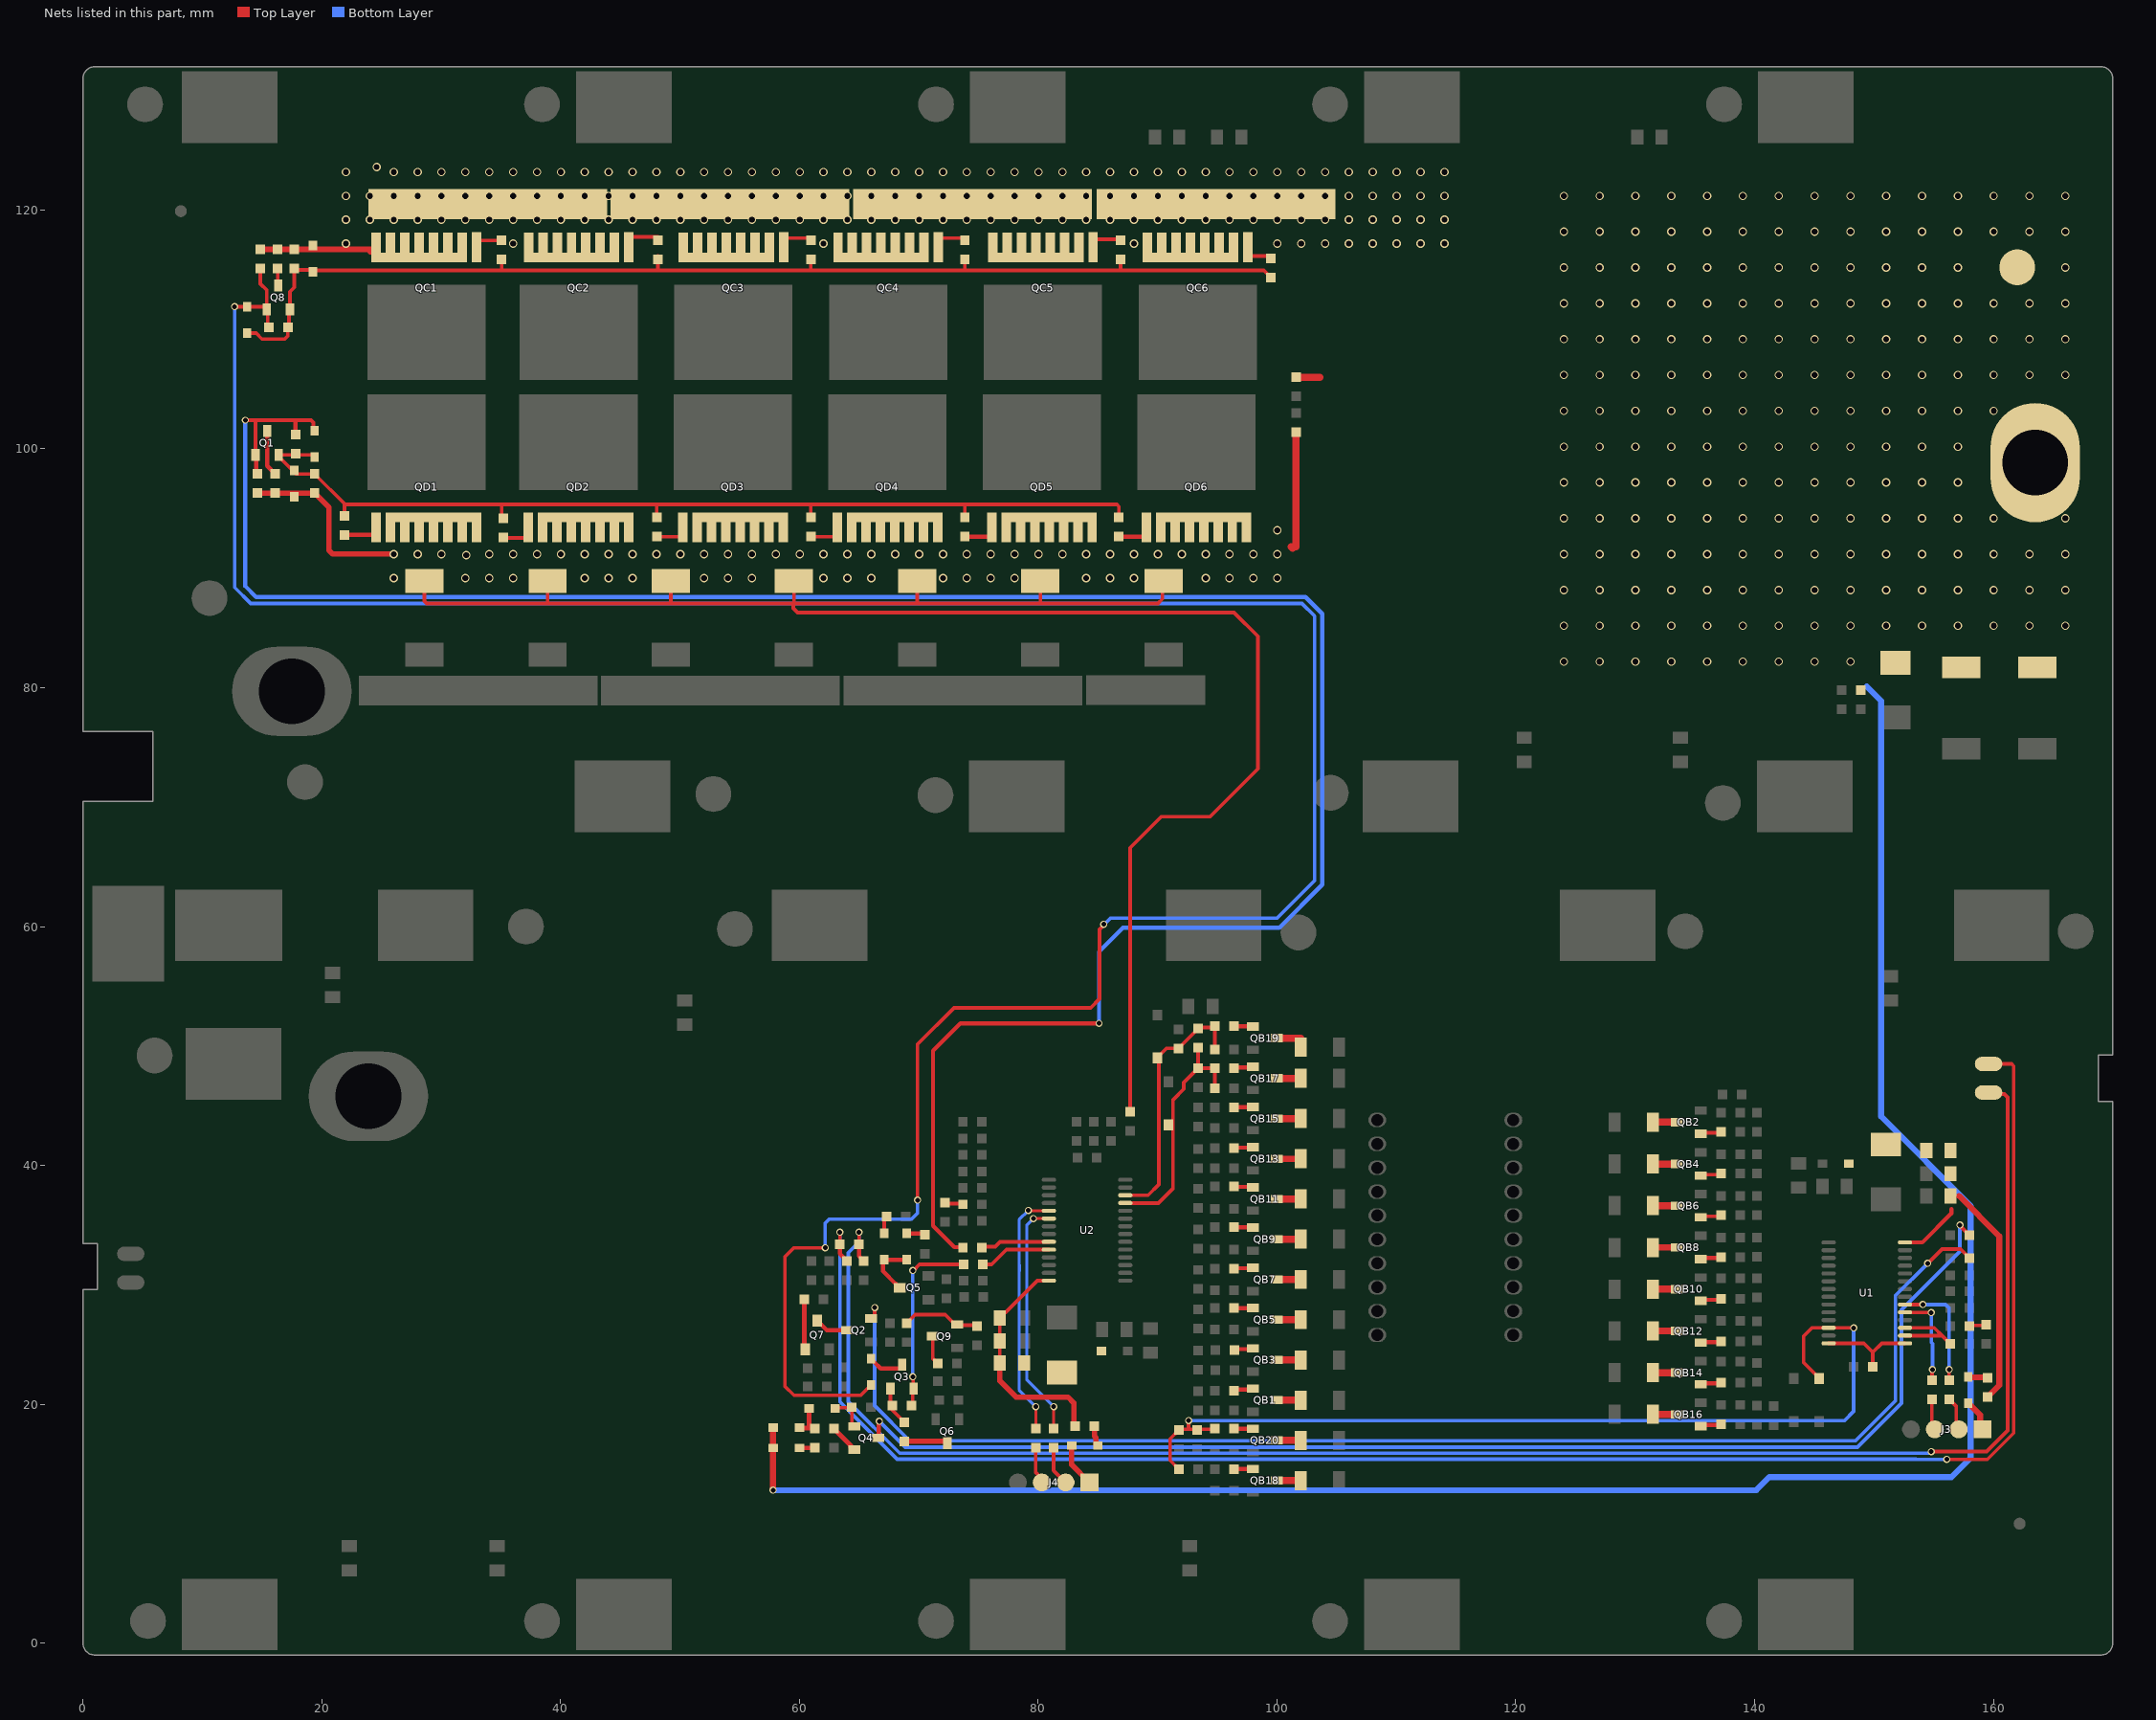
[diagram p0: the nets of this part, all layers, seen from the top]
# Altium PCB MISC82749.PcbDoc (part 3 of 4)
Units mm, origin at the board's own origin, x right, y up, seen from the top; angles counter-clockwise.
Board outline 170 x 133 mm, 2 copper layers (Top Layer, Bottom Layer); 262 components, 170 nets, 783 pads, 1052 vias.

## Via types
v1: diameter 0.7, hole 0.5, Top Layer to Bottom Layer, tented both sides, 953 vias
v2: diameter 0.6, hole 0.4, Top Layer to Bottom Layer, tented both sides, 99 vias

## Nets (pads, with @x,y where several pads share a name; then routed paths per layer and width w, separated by ;. In a path a pad name is that pad's centre, name@x,y a point inside that pad or via, vN(x,y) a via of type N, cw(c..) or ccw(c..) an arc to the next point about the centre after c; other vN are vias at no path point) (continued)
NetC45_2: C45.2 QD1.2 QD2.2 QD3.2 QD4.2 QD5.2 QD6.2 R30.2 R40.2 R41.2 R43.2 RS1.2 RS2.2 RS3.2 RS4.2 RS5.2 RS6.2 RS7.2 Z1.2 | length 186.9
  Top Layer w0.3: RS7.2@28.6,88.95 28.6,87.255 28.805,87.05 39.053,87.05 ; RS6.2@38.917,88.95 38.917,87.186 39.053,87.05 ; RS5.2@49.233,88.95 49.233,87.117 49.3,87.05 ; RS4.2@59.55,88.95 59.55,87.1 59.5,87.05 ; RS3.2@69.867,88.95 69.867,87.183 70,87.05 ; RS2.2@80.183,88.95 80.183,87.067 80.2,87.05 ; R30.2@87.7,44.5 87.7,66.593 90.307,69.2 94.4,69.2 98.4,73.2 98.4,84.3 96.4,86.3 59.85,86.3 59.5,86.65 59.5,87.05 ; RS1.2@90.5,88.95 90.407,88.857 90.407,87.428 90.03,87.05 80.2,87.05 ; 39.053,87.05 49.3,87.05 ; 49.3,87.05 59.5,87.05 ; 59.5,87.05 70,87.05 ; 70,87.05 80.2,87.05
  Top Layer w0.45: R40.2@14.6,96.3 R41.2@16.1,96.3 R43.2@19.4,96.3 20.6,95.1 20.6,91.5 20.9,91.2 v1@25.7,91.2
  Top Layer w0.6: 101.2,91.8 101.3,91.7 ; 101.6,91.8 C45.2@101.6,101.4
  other v1: 26.027,89.182 32.028,89.182 34.028,89.182 36.028,89.182 42.028,89.182 44.028,89.182 46.028,89.182 52.028,89.182 54.028,89.182 56.028,89.182 62.028,89.182 64.028,89.182 66.028,89.182 72.028,89.182 74.028,89.182 76.028,89.182 78.028,89.182 84.028,89.182 86.028,89.182 88.028,89.182 94.028,89.182 96.028,89.182 98.028,89.182 100.028,89.182 32.1,91.1 26.027,91.182 28.027,91.182 30.027,91.182 34.028,91.182 36.028,91.182 38.028,91.182 40.028,91.182 42.028,91.182 44.028,91.182 46.028,91.182 48.028,91.182 50.028,91.182 52.028,91.182 54.028,91.182 56.028,91.182 58.028,91.182 60.028,91.182 62.028,91.182 64.028,91.182 66.028,91.182 68.028,91.182 70.028,91.182 72.028,91.182 74.028,91.182 76.028,91.182 78.028,91.182 80.028,91.182 82.028,91.182 84.028,91.182 86.028,91.182 88.028,91.182 90.028,91.182 92.028,91.182 94.028,91.182 96.028,91.182 98.028,91.182 100.028,91.182 100.028,93.182
NetD1_1: D1.1 R26.2 TVS1.1
NetD2_1: D2.1 R27.2 TVS2.1
NetD7_1: D7.1 R34.2 | length 1.5
  Top Layer w0.5: D7.1@157.95,22.25 R34.2@159.45,22.25
NetD7_2: D7.2 J3.1 | length 2.7
  Top Layer w0.5: D7.2@157.9,20.1 157.9,20.05 158,19.95 158.05,19.95 158.893,19.107 158.893,18.057 J3.1@159.05,17.9
NetD8_1: D8.1 R37.2 | length 1.7
  Top Layer w0.45: R37.2@84.7,18.15 84.711,18.139 84.711,17.339 84.848,17.202 84.848,16.675 84.973,16.55 D8.1@85,16.55
NetD8_2: D8.2 J4.1 | length 3.7
  Top Layer w0.45: D8.2@82.8,16.55 82.8,14.95 J4.1@84.3,13.45
NetD11_1: D11.1 Q1.2 R42.2 R43.1 RD1.1 RD2.1 RD3.1 RD4.2 RD5.2 RD6.2 Z1.1 | length 82
  Top Layer w0.3: R42.2@17.8,99.6 R42.2@17.9,99.5 ; D11.1@19.4,99.3 19.2,99.5 R42.2@17.9,99.5 ; RD1.1@21.9,94.4 21.9,95.35 ; RD2.1@35.06,94.15 35.06,95.29 35,95.35 ; RD3.1@48.06,94.25 48.06,95.31 48.1,95.35 ; RD4.2@60.96,94.25 60.96,95.31 61,95.35 ; RD5.2@73.86,94.25 73.86,95.29 73.8,95.35 ; RD6.2@86.76,94.25 86.76,95.174 86.584,95.35 73.8,95.35 ; R42.2@17.9,99.5 Q1.2@16.4,99.5 16.4,99.35 17.85,97.9 R43.1@19.4,97.9 21.9,95.4 21.9,95.35 ; 21.9,95.35 35,95.35 ; 35,95.35 48.1,95.35 ; 48.1,95.35 61,95.35 ; 61,95.35 73.8,95.35
NetD11_2: D11.2 Q1.1 R33.2 R40.1 R42.1 | length 199.7
  Top Layer w0.35: v2(13.6,102.4) 17.8,102.4 ; 14.45,102.3 Q1.1@14.45,99.5 14.525,99.425 14.525,97.975 R40.1@14.6,97.9 ; R42.1@17.8,101.2 17.8,102.4 ; D11.2@19.4,101.5 19.303,101.597 19.303,102.195 19.097,102.4 17.8,102.4 ; R33.2@73.7,33.1 73.649,33.151 72.98,33.151 71.2,34.931 71.2,49.6 73.5,51.9 v2(85.1,51.9)
  Bottom Layer w0.35: v2(13.6,102.4) 13.6,88.5 14.5,87.6 102.4,87.6 103.8,86.2 103.8,63.5 100.2,59.9 87.1,59.9 85.1,57.9 v2(85.1,51.9)
NetD12_1: D12.1 D13.2 Q8.1 R53.1 R65.1 | length 234.2
  Top Layer w0.3: v2(12.7,111.9) 12.704,111.896 13.756,111.896 D13.2@13.76,111.892 15.185,111.892 Q8.1@15.385,111.692 ; R65.1@14.86,115.1 14.86,113.825 15.385,113.3 Q8.1@15.385,111.692 ; R53.1@15.56,110.192 15.472,110.279 15.472,111.588 Q8.1@15.385,111.676 Q8.1@15.385,111.692 ; v2(62.164,33.1) 59.538,33.1 58.8,32.362 58.8,21.5 59.55,20.75 65.15,20.75 65.75,21.35 65.8,21.35 66,21.55 D12.1@66,21.6 ; v2(69.9,37.1) 69.9,50.15 72.95,53.2 84.4,53.2 85.15,53.95 85.15,59.769 85.5,60.119 v2(85.5,60.2)
  Bottom Layer w0.3: v2(12.7,111.9) 12.7,88.4 14.05,87.05 102.1,87.05 103.15,86 103.15,63.85 100,60.7 86.061,60.7 85.561,60.2 v2(85.5,60.2) ; v2(62.164,33.1) 62.164,35.164 62.5,35.5 69.4,35.5 69.9,36 v2(69.9,37.1)
NetD12_2: D12.2 Q3.3 | length 3.2
  Top Layer w0.35: D12.2@66,23.8 66,23.75 66.175,23.575 66.225,23.575 66.8,23 68.425,23 68.6,23.175 Q3.3@68.6,23.316
NetD13_1: D13.1 Q8.2 R52.1 R53.2 RC1.1 RC2.2 RC3.2 RC4.1 RC5.1 RC6.1 Z3.1 | length 97.1
  Top Layer w0.3: D13.1@13.76,109.692 14.508,109.692 15,109.2 16.9,109.2 17.16,109.46 R53.2@17.16,110.192 17.247,110.279 17.247,111.588 Q8.2@17.335,111.676 17.335,113.155 17.7,113.52 R52.1@17.7,115.1 17.81,114.99 Z3.1@19.26,114.99 ; Z3.1@19.26,114.842 19.368,114.95 35.1,114.95 ; RC1.1@35.06,115.85 35.06,114.99 35.1,114.95 ; RC2.2@48.16,116.15 48.16,114.99 48.2,114.95 ; RC3.2@60.96,116.05 60.96,115.01 60.9,114.95 ; RC4.1@73.86,116.05 73.86,114.99 73.9,114.95 ; RC5.1@86.9,115.95 86.9,115.05 86.8,114.95 ; RC6.1@99.5,114.35 98.9,114.95 86.8,114.95 ; 35.1,114.95 48.2,114.95 ; 48.2,114.95 60.9,114.95 ; 60.9,114.95 73.9,114.95 ; 73.9,114.95 86.8,114.95
NetD14_1: D14.1 R55.1 | length 1.5
  Top Layer w0.35: D14.1@69,34.3 70.275,34.3 70.35,34.225 R55.1@70.35,34.1
NetD14_2: D14.2 D16.1 Q5.3 | length 4.8
  Top Layer w0.35: Q5.3@68.4,29.75 68.3,29.75 68.075,29.975 68.075,30.075 67,31.15 67,32.1 D16.1@67.1,32.1 D14.2@68.8,32.1
NetD15_2: D15.2 R58.1 Z2.2 | length 3
  Top Layer w0.4: D15.2@60,18.05 60.05,18 60.7,18 ; Z2.2@60.8,19.65 60.8,18.1 60.7,18 ; R58.1@61.3,17.95 61.25,18 60.7,18
NetD16_2: D16.2 R66.2 | length 1.4
  Top Layer w0.3: D16.2@67.1,34.3 R66.2@67.1,35.7
NetD17_2: D17.2 R57.1 | length 1.3
  Top Layer w0.35: D17.2@60,16.35 R57.1@61.3,16.35
NetJ3_2: J3.2 R35.2 | length 2.8
  Top Layer w0.3: R35.2@156.3,20.4 156.9,19.8 156.9,18.1 J3.2@157.1,17.9
NetJ3_3: J3.3 R36.2 | length 2.6
  Top Layer w0.3: R36.2@154.85,20.4 154.85,18.475 155.1,18.225 J3.3@155.1,17.9
NetJ4_2: J4.2 R38.2 | length 3.3
  Top Layer w0.3: R38.2@81.3,16.35 81.3,14.45 J4.2@82.3,13.45
NetJ4_3: J4.3 R39.2 | length 3.1
  Top Layer w0.3: R39.2@79.8,16.35 79.8,14.275 80.3,13.775 J4.3@80.3,13.45
NetQ1_3: Q1.3 R41.1 | length 3.9
  Top Layer w0.35: Q1.3@15.425,101.516 15.425,98.575 R41.1@16.1,97.9
NetQ2_2: Q2.2 R44.1 | length 114.3
  Top Layer w0.3: Q2.2@66,27.175 66.11,27.175 66.31,27.375 v2(66.31,28.09) ; v2(154.5,31.8) 155.7,33 157.25,33 R44.1@158,32.25
  Bottom Layer w0.3: v2(66.31,28.09) 66.31,19.883 69.243,16.95 148.457,16.95 151.8,20.293 151.8,29.1 v2(154.5,31.8)
NetQ2_3: Q2.3 Q7.3 | length 2.7
  Top Layer w0.35: Q7.3@61.5,27 61.5,26.9 61.725,26.675 61.825,26.675 62.3,26.2 Q2.3@63.8,26.2
NetQ3_1: Q3.1 R54.1 R56.1 | length 3.3
  Top Layer w0.3: Q3.1@67.625,21.3 67.625,19.675 R56.1@68.8,18.5
NetQ3_2: Q3.2 R32.2 R54.2 | length 15.8
  Top Layer w0.3: R54.2@69.4,19.9 69.488,19.988 69.488,21.388 69.538,21.438 69.538,22.263 v2(69.5,22.3) ; v2(69.5,31.2) 69.542,31.2 70.051,31.71 R32.2@73.76,31.71
  Bottom Layer w0.3: v2(69.5,22.3) v2(69.5,31.2)
NetQ4_1: Q4.1 R45.2 Z2.1 | length 3.1
  Top Layer w0.3: Z2.1@63,19.65 63.05,19.7 64.35,19.7 R45.2@64.4,19.75 64.4,18.35 Q4.1@64.6,18.15
NetQ4_2: Q4.2 R58.2 | length 2.5
  Top Layer w0.4: R58.2@62.9,17.95 64.3,16.55 64.3,16.35 64.45,16.2 Q4.2@64.6,16.2
NetQ4_3: Q4.3 R48.1 | length 107.6
  Top Layer w0.3: v2(157.2,35) 157.2,34.95 R48.1@158,34.15
  Top Layer w0.35: Q4.3@66.616,17.175 66.658,17.217 66.658,18.532 v2(66.7,18.574)
  Bottom Layer w0.3: v2(66.7,18.574) 68.874,16.4 148.614,16.4 152.3,20.086 152.3,27.9 157.2,32.8 v2(157.2,35)
NetQ6_3: Q6.3 R56.2 | length 3.7
  Top Layer w0.45: R56.2@68.815,16.9 72.275,16.9 72.4,16.775 Q6.3@72.4,16.734
NetQ7_1: Q7.1 R50.1 | length 3.7
  Top Layer w0.4: 60.4,25.144 R50.1@60.4,28.8
NetQ8_3: Q8.3 R61.1 | length 1.4
  Top Layer w0.3: R61.1@16.28,115.1 16.32,115.06 16.32,113.732 Q8.3@16.36,113.692
NetQ9_2: Q9.2 R59.1 R64.1 | length 6.6
  Top Layer w0.3: R59.1@69,26.8 69.7,27.5 72.225,27.5 73.05,26.675 Q9.2@73.2,26.675 ; Q9.2@73.2,26.613 74.838,26.613 R64.1@74.9,26.55
NetQ9_3: Q9.3 R62.2 | length 2.5
  Top Layer w0.3: Q9.3@71.184,25.7 71.184,23.816 R62.2@71.6,23.4
NetQB1_1: QB1.1 RB3.1 | length 1.7
  Top Layer w0.35: RB3.1@96.4,21.15 96.485,21.235 97.899,21.235 QB1.1@97.984,21.32
NetQB1_3: QB1.3 RB1.2 | length 2
  Top Layer w0.6: QB1.3@100,20.345 RB1.2@102,20.345
NetQB2_1: QB2.1 RB4.1 | length 1.8
  Top Layer w0.35: QB2.1@135.5,42.643 135.587,42.73 137.113,42.73 RB4.1@137.2,42.818
NetQB2_3: QB2.3 RB2.2 | length 2
  Top Layer w0.6: RB2.2@131.484,43.618 QB2.3@133.484,43.618
NetQB3_1: QB3.1 RB7.1 | length 1.6
  Top Layer w0.35: RB7.1@96.45,24.55 96.519,24.619 97.915,24.619 QB3.1@97.984,24.689
NetQB3_3: QB3.3 RB5.2 | length 2
  Top Layer w0.6: QB3.3@100,23.714 RB5.2@102,23.714
NetQB4_1: QB4.1 RB8.1 | length 1.8
  Top Layer w0.3: QB4.1@135.5,39.147 135.586,39.233 137.114,39.233 RB8.1@137.2,39.32
NetQB4_3: QB4.3 RB6.2 | length 2
  Top Layer w0.6: RB6.2@131.484,40.122 QB4.3@133.484,40.122
NetQB5_1: QB5.1 RB11.1 | length 1.6
  Top Layer w0.35: RB11.1@96.4,28.05 96.403,28.053 97.981,28.053 QB5.1@97.984,28.057
NetQB5_3: QB5.3 RB9.2 | length 2
  Top Layer w0.6: QB5.3@100,27.082 RB9.2@102,27.082
NetQB6_1: QB6.1 RB12.1 | length 1.8
  Top Layer w0.3: QB6.1@135.5,35.652 135.585,35.737 137.115,35.737 RB12.1@137.2,35.822
NetQB6_3: QB6.3 RB10.2 | length 2
  Top Layer w0.6: RB10.2@131.484,36.627 QB6.3@133.484,36.627
NetQB7_1: QB7.1 RB15.1 | length 1.6
  Top Layer w0.35: RB15.1@96.4,31.35 96.438,31.388 97.947,31.388 QB7.1@97.984,31.425
NetQB7_3: QB7.3 RB13.2 | length 2
  Top Layer w0.6: QB7.3@100,30.45 RB13.2@102,30.45
NetQB8_1: QB8.1 RB16.1 | length 1.8
  Top Layer w0.35: QB8.1@135.5,32.156 135.584,32.24 137.116,32.24 RB16.1@137.2,32.324
NetQB8_3: QB8.3 RB14.2 | length 2
  Top Layer w0.5: RB14.2@131.484,33.131 QB8.3@133.484,33.131
NetQB9_1: QB9.1 RB19.1 | length 1.6
  Top Layer w0.35: RB19.1@96.4,34.85 96.428,34.822 97.956,34.822 QB9.1@97.984,34.793
NetQB9_3: QB9.3 RB17.2 | length 2
  Top Layer w0.6: QB9.3@100,33.818 RB17.2@102,33.818
NetQB10_1: QB10.1 RB20.1 | length 1.8
  Top Layer w0.35: QB10.1@135.5,28.661 135.582,28.744 137.118,28.744 RB20.1@137.2,28.826
NetQB10_3: QB10.3 RB18.2 | length 2
  Top Layer w0.6: RB18.2@131.484,29.636 QB10.3@133.484,29.636
NetQB11_1: QB11.1 RB23.1 | length 1.6
  Top Layer w0.35: RB23.1@96.4,38.25 96.444,38.206 97.94,38.206 QB11.1@97.984,38.161
NetQB11_3: QB11.3 RB21.2 | length 2
  Top Layer w0.6: QB11.3@100,37.186 RB21.2@102,37.186
NetQB12_1: QB12.1 RB24.1 | length 1.7
  Top Layer w0.35: QB12.1@135.5,25.166 135.542,25.208 137.158,25.208 RB24.1@137.2,25.25
NetQB12_3: QB12.3 RB22.2 | length 2
  Top Layer w0.6: RB22.2@131.484,26.141 QB12.3@133.484,26.141
NetQB13_1: QB13.1 RB27.1 | length 1.6
  Top Layer w0.35: RB27.1@96.4,41.45 96.44,41.49 97.944,41.49 QB13.1@97.984,41.53
NetQB13_3: QB13.3 RB25.2 | length 2
  Top Layer w0.5: QB13.3@100,40.555 RB25.2@102,40.555
NetQB14_1: QB14.1 RB28.1 | length 1.8
  Top Layer w0.35: QB14.1@135.5,21.67 135.58,21.75 137.12,21.75 RB28.1@137.2,21.83
NetQB14_3: QB14.3 RB26.2 | length 2
  Top Layer w0.6: RB26.2@131.484,22.645 QB14.3@133.484,22.645
NetQB15_1: QB15.1 RB31.1 | length 1.6
  Top Layer w0.35: RB31.1@96.4,44.85 96.424,44.874 97.96,44.874 QB15.1@97.984,44.898
NetQB15_3: QB15.3 RB29.2 | length 2
  Top Layer w0.6: QB15.3@100,43.923 RB29.2@102,43.923
NetQB16_1: QB16.1 RB32.1 | length 1.8
  Top Layer w0.35: QB16.1@135.5,18.175 135.579,18.254 137.121,18.254 RB32.1@137.2,18.332
NetQB16_3: QB16.3 RB30.2 | length 2
  Top Layer w0.6: RB30.2@131.484,19.15 QB16.3@133.484,19.15
NetQB17_1: QB17.1 RB35.1 | length 1.6
  Top Layer w0.35: RB35.1@96.4,48.15 96.458,48.208 97.926,48.208 QB17.1@97.984,48.266
NetQB17_3: QB17.3 RB33.2 | length 2
  Top Layer w0.6: QB17.3@100,47.291 RB33.2@102,47.291
NetQB18_1: QB18.1 RB36.1 | length 1.6
  Top Layer w0.35: RB36.1@96.4,14.55 96.417,14.567 97.967,14.567 QB18.1@97.984,14.584
NetQB18_3: QB18.3 RB34.2 | length 2
  Top Layer w0.6: QB18.3@100,13.609 RB34.2@102,13.609
NetQB19_1: QB19.1 RB39.1 | length 1.6
  Top Layer w0.3: RB39.1@96.4,51.5 RB39.1@96.467,51.567
  Top Layer w0.35: RB39.1@96.467,51.567 96.542,51.642 97.976,51.642 QB19.1@97.984,51.634
NetQB19_3: QB19.3 RB37.2 | length 2
  Top Layer w0.6: QB19.3@100,50.659 RB37.2@102,50.659
NetQB20_1: QB20.1 RB40.1 | length 1.6
  Top Layer w0.35: RB40.1@96.4,17.95 96.401,17.951 97.983,17.951 QB20.1@97.984,17.952
NetQB20_3: QB20.3 RB38.2 | length 2
  Top Layer w0.6: QB20.3@100,16.977 RB38.2@102,16.977
NetQC1_1: QC1.1 RC1.2 | length 2.7
  Top Layer w0.3: QC1.1@32.76,116.888 32.76,117.2 33.01,117.45 RC1.2@35.06,117.45
NetQC2_1: QC2.1 RC2.1 | length 3.2
  Top Layer w0.3: QC2.1@45.72,116.888 45.72,117.5 45.97,117.75 RC2.1@48.16,117.75
NetQC3_1: QC3.1 RC3.1 | length 2.9
  Top Layer w0.3: QC3.1@58.68,116.888 58.68,117.4 58.93,117.65 RC3.1@60.96,117.65
NetQC4_1: QC4.1 RC4.2 | length 2.8
  Top Layer w0.3: QC4.1@71.64,116.888 71.64,117.4 71.89,117.65 RC4.2@73.86,117.65
NetQC5_1: QC5.1 RC5.2 | length 2.8
  Top Layer w0.3: QC5.1@84.6,116.888 84.6,117.3 84.85,117.55 RC5.2@86.9,117.55
NetQC6_1: QC6.1 RC6.2 | length 2.1
  Top Layer w0.35: QC6.1@97.492,116.15 99.3,116.15 RC6.2@99.5,115.95
NetQD1_1: QD1.1 RD1.2 | length 3.2
  Top Layer w0.3: QD1.1@24.36,93.35 QD1.1@24.36,93.412
  Top Layer w0.35: RD1.2@21.9,92.8 24.335,92.8 24.56,93.025 QD1.1@24.56,93.412
NetQD2_1: QD2.1 RD2.2 | length 3
  Top Layer w0.3: RD2.2@35.06,92.55 37.05,92.55 37.3,92.8 QD2.1@37.3,93.412
NetQD3_1: QD3.1 RD3.2 | length 2.8
  Top Layer w0.3: RD3.2@48.06,92.65 49.99,92.65 50.24,92.9 QD3.1@50.24,93.412
NetQD4_1: QD4.1 RD4.1 | length 2.8
  Top Layer w0.3: RD4.1@60.96,92.65 62.93,92.65 63.18,92.9 QD4.1@63.18,93.412
NetQD5_1: QD5.1 RD5.1 | length 2.9
  Top Layer w0.35: RD5.1@73.86,92.65 75.895,92.65 76.12,92.875 QD5.1@76.12,93.412
NetQD6_1: QD6.1 RD6.1 | length 2.9
  Top Layer w0.35: RD6.1@86.76,92.65 88.835,92.65 89.06,92.875 QD6.1@89.06,93.412
NetR28_2: R28.2 U1.14 U1.15 | length 8.2
  Top Layer w0.3: U1.14@146.2,25.1 149.15,25.1 149.9,24.35 ; R28.2@149.9,23.15 149.9,24.35 ; U1.15@152.6,25.1 150.65,25.1 149.9,24.35
NetR32_1: R32.1 U2.24 | length 6.4
  Top Layer w0.3: R32.1@75.619,31.45 R32.1@75.36,31.71 76.11,31.71 77.35,32.95 U2.24@80.9,32.95
NetR33_1: R33.1 U2.23 | length 5.8
  Top Layer w0.3: R33.1@75.3,33.1 75.4,33.2 76.4,33.2 76.8,33.6 U2.23@80.9,33.6
NetR67_1: R67.1 R70.2 SW1.1 | length 146.8
  Top Layer w0.254: R67.1@65.4,32 R67.1@65.627,31.773
  Top Layer w0.3: R70.2@65,33.4 v2(65,34.4) ; v2(154.8,16.038) 159.438,16.038 161.2,17.8 161.2,45.7 160.917,45.983 159.717,45.983 SW1.1@159.6,46.1
  Top Layer w0.35: R70.2@65,33.4 65,32.4 R67.1@65.4,32
  Bottom Layer w0.3: v2(65,34.4) 65,33.6 64.1,32.7 64.1,20.207 68.407,15.9 154.581,15.9 154.719,16.038 v2(154.8,16.038)
NetR68_2: R68.2 R70.1 SW1.2 | length 151
  Top Layer w0.3: R70.1@63.4,33.4 v2(63.4,34.4) ; v2(156.1,15.388) 156.088,15.4 156.1,15.4 156.112,15.388 159.495,15.388 161.7,17.593 161.7,48.324 161.524,48.5 SW1.2@159.6,48.5
  Top Layer w0.35: R70.1@63.4,33.4 63.4,32.6 R68.2@64,32
  Bottom Layer w0.3: v2(63.4,34.4) 63.4,20.2 64.95,18.65 64.95,18.643 68.193,15.4 153.5,15.4 153.512,15.388 v2(156.1,15.388)
NetR71_2: R71.2 U1.16 U1.17 | length 7.5
  Top Layer w0.3: U1.16@152.6,25.75 155.7,25.75 ; U1.17@152.6,26.4 155.05,26.4 155.7,25.75 ; R71.2@156.4,25.05 155.7,25.75
NetRT5_1: RT5.1 RT7.1 | length 1.4
  Top Layer w0.3: RT7.1@158,26.55 158.05,26.6 159.35,26.6 RT5.1@159.4,26.65
NetRT6_1: RT6.1 RT8.1 | length 1.5
  Top Layer w0.3: RT6.1@72.256,36.805 73.635,36.805 RT8.1@73.7,36.74
P-/C-: C41.1 C46.1 D9.2 D15.1 D17.1 pad.66@163.5,98.85 pad.82@33.9,120.5 pad.83@54.2,120.5 pad.84 pad.85 pad.86@162,115.2 QC1.2 QC2.2 QC3.2 QC4.2 QC5.2 QC6.2 R52.2 R61.2 R65.2 TVS3.1 TVS4.1 Z3.2 | length 188.7
  Top Layer w0.5: R65.2@14.86,116.7 R61.2@16.28,116.7 R52.2@17.7,116.7 24.41,116.7 24.56,116.85 QC1.2@24.56,117.25 ; 24.068,116.508 24.21,116.65 QC1.2@24.41,116.65 ; v2(57.8,12.8) D17.1@57.8,16.35 D15.1@57.8,18.05 ; C46.1@101.6,106 C46.1@101.75,106.15 ; D9.2@151.05,82.85 D9.2@151.8,82.1
  Top Layer w0.6: C46.1@101.6,106 103.2,106 103.6,106
  Bottom Layer w0.5: v2(57.8,12.8) 140.139,12.8 141.239,13.9 156.5,13.9 158.1,15.5 158.1,36.6 150.6,44.1 150.6,78.9 149.4,80.1
  other v1: 124.027,82.182 127.027,82.182 130.027,82.182 133.027,82.182 136.027,82.182 139.027,82.182 142.027,82.182 145.027,82.182 148.027,82.182 124.027,85.182 127.027,85.182 130.027,85.182 133.027,85.182 136.027,85.182 139.027,85.182 142.027,85.182 145.027,85.182 148.027,85.182 151.027,85.182 154.027,85.182 157.027,85.182 160.027,85.182 163.027,85.182 166.027,85.182 124.027,88.182 127.027,88.182 130.027,88.182 133.027,88.182 136.027,88.182 139.027,88.182 142.027,88.182 145.027,88.182 148.027,88.182 151.027,88.182 154.027,88.182 157.027,88.182 160.027,88.182 163.027,88.182 166.027,88.182 124.027,91.182 127.027,91.182 130.027,91.182 133.027,91.182 136.027,91.182 139.027,91.182 142.027,91.182 145.027,91.182 148.027,91.182 151.027,91.182 154.027,91.182 157.027,91.182 160.027,91.182 163.027,91.182 166.027,91.182 124.027,94.182 127.027,94.182 130.027,94.182 133.027,94.182 136.027,94.182 139.027,94.182 142.027,94.182 145.027,94.182 148.027,94.182 151.027,94.182 154.027,94.182 157.027,94.182 160.027,94.182 166.027,94.182 124.027,97.182 127.027,97.182 130.027,97.182 133.027,97.182 136.027,97.182 139.027,97.182 142.027,97.182 145.027,97.182 148.027,97.182 151.027,97.182 154.027,97.182 157.027,97.182 124.027,100.182 127.027,100.182 130.027,100.182 133.027,100.182 136.027,100.182 139.027,100.182 142.027,100.182 145.027,100.182 148.027,100.182 151.027,100.182 154.027,100.182 157.027,100.182 124.027,103.182 127.027,103.182 130.027,103.182 133.027,103.182 136.027,103.182 139.027,103.182 142.027,103.182 145.027,103.182 148.027,103.182 151.027,103.182 154.027,103.182 157.027,103.182 160.027,103.182 124.027,106.182 127.027,106.182 130.027,106.182 133.027,106.182 136.027,106.182 139.027,106.182 142.027,106.182 145.027,106.182 148.027,106.182 151.027,106.182 154.027,106.182 157.027,106.182 160.027,106.182 163.027,106.182 166.027,106.182 124.027,109.182 127.027,109.182 130.027,109.182 133.027,109.182 136.027,109.182 139.027,109.182 142.027,109.182 145.027,109.182 148.027,109.182 151.027,109.182 154.027,109.182 157.027,109.182 160.027,109.182 163.027,109.182 166.027,109.182 124.027,112.182 127.027,112.182 130.027,112.182 133.027,112.182 136.027,112.182 139.027,112.182 142.027,112.182 145.027,112.182 148.027,112.182 151.027,112.182 154.027,112.182 157.027,112.182 160.027,112.182 163.027,112.182 166.027,112.182 124.027,115.182 127.027,115.182 130.027,115.182 133.027,115.182 136.027,115.182 139.027,115.182 142.027,115.182 145.027,115.182 148.027,115.182 151.027,115.182 154.027,115.182 157.027,115.182 166.027,115.182 22.027,117.182 36.028,117.182 62.028,117.182 88.028,117.182 100.028,117.182 102.028,117.182 104.028,117.182 106.028,117.182 108.028,117.182 110.028,117.182 112.028,117.182 114.028,117.182 124.027,118.182 127.027,118.182 130.027,118.182 133.027,118.182 136.027,118.182 139.027,118.182 142.027,118.182 145.027,118.182 148.027,118.182 151.027,118.182 154.027,118.182 157.027,118.182 160.027,118.182 163.027,118.182 166.027,118.182 22.027,119.182 24.027,119.182 26.027,119.182 28.027,119.182 30.027,119.182 32.028,119.182 34.028,119.182 36.028,119.182 38.028,119.182 40.028,119.182 42.028,119.182 44.028,119.182 46.028,119.182 48.028,119.182 50.028,119.182 52.028,119.182 54.028,119.182 56.028,119.182 58.028,119.182 60.028,119.182 62.028,119.182 64.028,119.182 66.028,119.182 68.028,119.182 70.028,119.182 72.028,119.182 74.028,119.182 76.028,119.182 78.028,119.182 80.028,119.182 82.028,119.182 84.028,119.182 86.028,119.182 88.028,119.182 90.028,119.182 92.028,119.182 94.028,119.182 96.028,119.182 98.028,119.182 100.028,119.182 102.028,119.182 104.028,119.182 106.028,119.182 108.028,119.182 110.028,119.182 112.028,119.182 114.028,119.182 22.027,121.182 24.027,121.182 26.027,121.182 28.027,121.182 30.027,121.182 32.028,121.182 34.028,121.182 36.028,121.182 38.028,121.182 40.028,121.182 42.028,121.182 44.028,121.182 46.028,121.182 48.028,121.182 50.028,121.182 52.028,121.182 54.028,121.182 56.028,121.182 58.028,121.182 60.028,121.182 62.028,121.182 64.028,121.182 66.028,121.182 68.028,121.182 70.028,121.182 72.028,121.182 74.028,121.182 76.028,121.182 78.028,121.182 80.028,121.182 82.028,121.182 84.028,121.182 86.028,121.182 88.028,121.182 90.028,121.182 92.028,121.182 94.028,121.182 96.028,121.182 98.028,121.182 100.028,121.182 102.028,121.182 104.028,121.182 106.028,121.182 108.028,121.182 110.028,121.182 112.028,121.182 114.028,121.182 124.027,121.182 127.027,121.182 130.027,121.182 133.027,121.182 136.027,121.182 139.027,121.182 142.027,121.182 145.027,121.182 148.027,121.182 151.027,121.182 154.027,121.182 157.027,121.182 160.027,121.182 163.027,121.182 166.027,121.182 22.027,123.182 26.027,123.182 28.027,123.182 30.027,123.182 32.028,123.182 34.028,123.182 36.028,123.182 38.028,123.182 40.028,123.182 42.028,123.182 44.028,123.182 46.028,123.182 48.028,123.182 50.028,123.182 52.028,123.182 54.028,123.182 56.028,123.182 58.028,123.182 60.028,123.182 62.028,123.182 64.028,123.182 66.028,123.182 68.028,123.182 70.028,123.182 72.028,123.182 74.028,123.182 76.028,123.182 78.028,123.182 80.028,123.182 82.028,123.182 84.028,123.182 86.028,123.182 88.028,123.182 90.028,123.182 92.028,123.182 94.028,123.182 96.028,123.182 98.028,123.182 100.028,123.182 102.028,123.182 104.028,123.182 106.028,123.182 108.028,123.182 110.028,123.182 112.028,123.182 114.028,123.182 24.6,123.6
RXD_M: R39.1 U2.19 | length 20.9
  Top Layer w0.254: v2(79.175,36.225) 79.187,36.213 80.888,36.213 U2.19@80.9,36.2 ; R39.1@79.8,17.95 v2(79.8,19.8)
  Bottom Layer w0.254: v2(79.175,36.225) 78.4,35.45 78.4,31.687 78.427,31.66 78.427,31.14 78.4,31.113 78.4,21.2 v2(79.8,19.8)
RXD_S: R36.1 U1.19 | length 7.9
  Top Layer w0.3: U1.19@152.6,27.7 152.61,27.69 154.785,27.69 v2(154.8,27.675) ; R36.1@154.85,22 154.875,22.025 154.875,22.875 v2(154.9,22.9)
  Bottom Layer w0.3: v2(154.8,27.675) 154.8,25.159 154.9,25.059 v2(154.9,22.9)
TXD_M: R38.1 U2.20 | length 20.1
  Top Layer w0.254: v2(79.604,35.55) U2.20@80.9,35.55 ; R38.1@81.3,17.95 v2(81.3,19.8)
  Bottom Layer w0.254: v2(79.604,35.55) 79.038,34.983 79.038,22.062 v2(81.3,19.8)
TXD_S: R35.1 U1.20 | length 9.9
  Top Layer w0.3: U1.20@152.6,28.35 v2(154.1,28.35) ; R35.1@156.3,22 v2(156.3,22.9)
  Bottom Layer w0.3: v2(154.1,28.35) 156,28.35 156.3,28.05 v2(156.3,22.9)
VBAT_M: C26.2 C29.2 R27.1 R37.1 U2.28 | length 19.7
  Top Layer w0.3: R27.1@76.794,23.46 C26.2@76.794,25.31 76.794,27.337 77.152,27.695 77.279,27.695 79.934,30.35 U2.28@80.9,30.35
  Top Layer w0.45: R27.1@76.794,23.46 76.794,21.956 78.15,20.6 82.5,20.6 83,20.1 83,18.25 R37.1@83.1,18.15
VBAT_S: C25.2 C28.2 R26.1 R34.1 U1.28 | length 23.9
  Top Layer w0.35: U1.28@152.6,33.55 154.058,33.55 156.5,35.992 156.5,36.35
  Top Layer w0.5: 157.12,37.45 160.5,34.07 160.5,21.6 R34.1@159.5,20.6
"VC0 M": C21.1 C22.2 D4.1 R22.2 RB39.2 U2.12 | length 21.6
  Top Layer w0.3: U2.12@87.3,37.5 89.2,37.5 90.1,38.4 D4.1@90.1,49 ; D4.1@90,49 90,49.05 90.75,49.8 C22.2@91.75,49.8 C21.1@93.4,51.45 93.5,51.55 94.7,51.55 RB39.2@94.8,51.65 R22.2@94.8,49.7
"VC0 S": C10.1 C11.2 D3.1 R11.2 RB40.2 U1.12 | length 79.3
  Top Layer w0.3: C10.1@91.8,14.55 91.05,15.3 91.05,17.1 R11.2@91.8,17.85 91.85,17.9 92.7,17.9 ; v2(92.6,18.63) 92.6,18 92.7,17.9 ; RB40.2@94.8,17.95 94.75,17.9 92.7,17.9 ; D3.1@145.4,22.2 144.1,23.5 144.1,25.7 144.8,26.4 v2(148.3,26.4)
  Bottom Layer w0.3: v2(92.6,18.63) 147.53,18.63 148.3,19.4 v2(148.3,26.4)
"VC1 M": C20.1 C21.2 D5.1 R21.2 RB35.2 U2.11 | length 20.2
  Top Layer w0.3: U2.11@87.3,36.85 90.068,36.85 91.3,38.082 91.3,45.5 92.2,46.4 92.2,46.95 C20.1@93.4,48.15 ; C21.2@93.4,49.85 C20.1@93.4,48.15 ; R21.2@94.8,46.45 RB35.2@94.8,48.15 C20.1@93.4,48.15